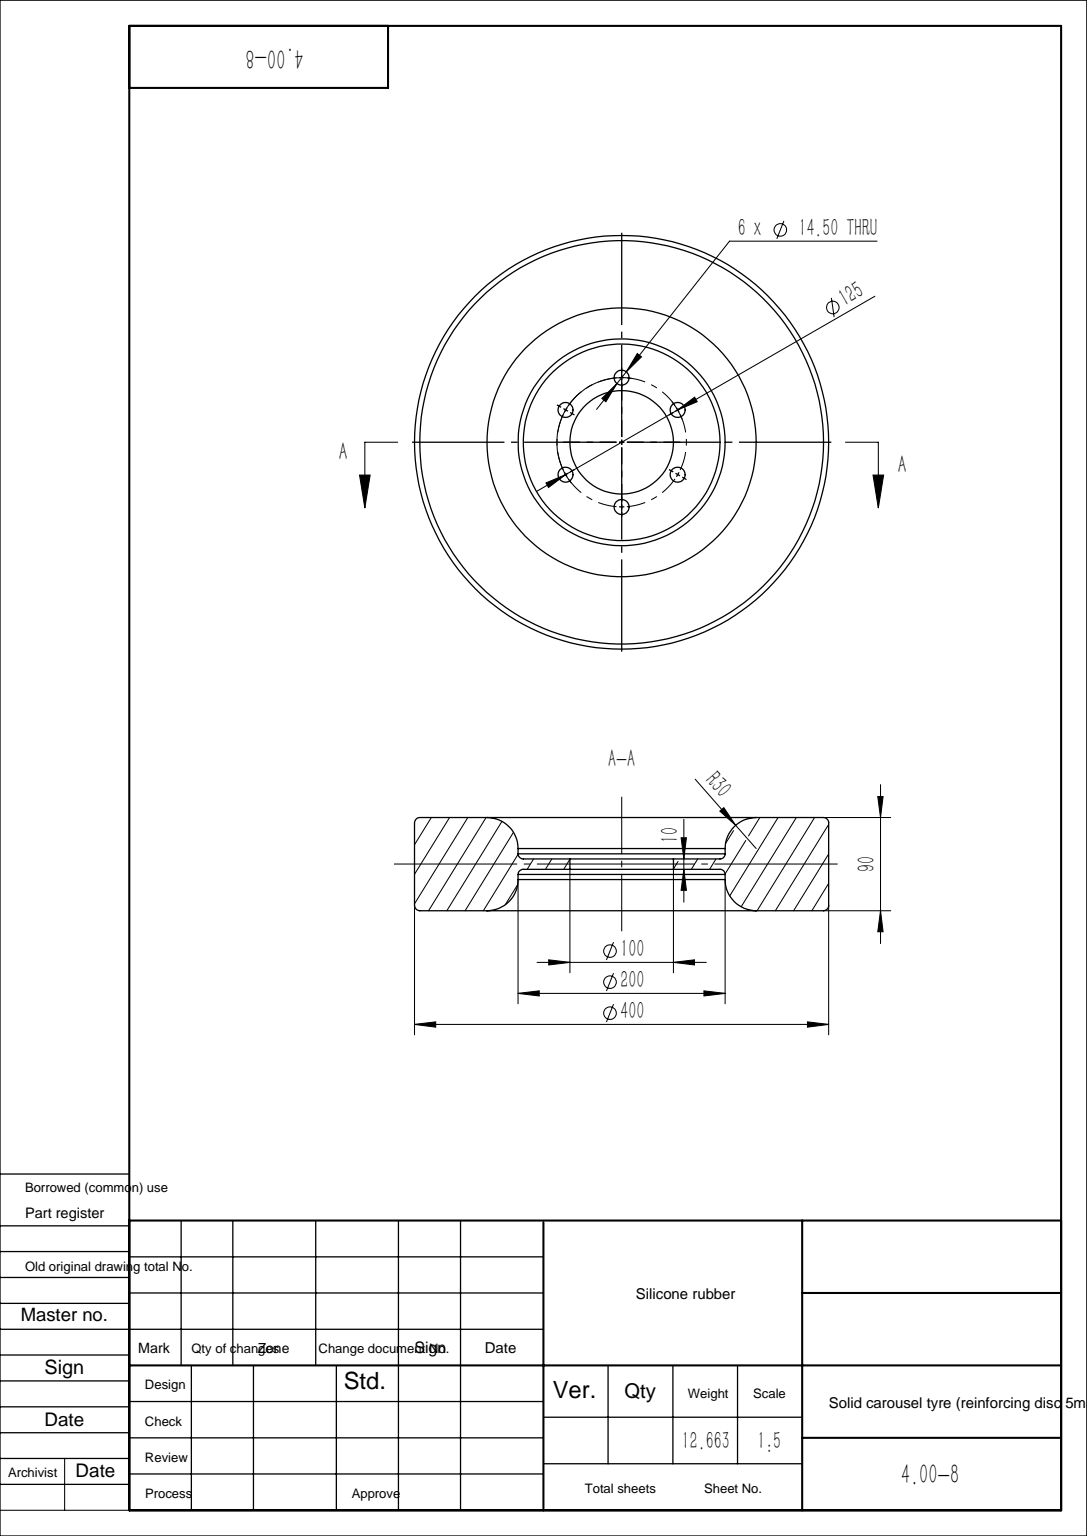
from build123d import *

# Parameters (mm, degrees)
FILLET1_R                    = 5
F_14_5_14_5_DIAMETER_HOLE1_D = 14.5


with BuildPart() as part:
    # Sketch2 → Revolve1 (revolve)
    with BuildSketch(Plane(origin=(0, 0, 0), x_dir=(1, 0, 0), z_dir=(0, 1, 0))):
        with BuildLine():
            Line((50, -5), (50, 5))
            Line((50, 5), (100, 5))
            Line((100, 5), (100, 15))
            ThreePointArc((100, 15), (108.786796564, 36.213203436), (130, 45))
            Line((130, 45), (200, 45))
            Line((200, 45), (200, -45))
            Line((200, -45), (130, -45))
            ThreePointArc((130, -45), (108.786796564, -36.213203436), (100, -15))
            Line((100, -15), (100, -5))
            Line((100, -5), (50, -5))
        make_face()
    revolve(axis=Axis((0, 0, 0), (0, 0, -1)))

    # Fillet1
    fillet1_edges = [part.edges().sort_by_distance(p)[0] for p in [
        (-100, 0, -5),
        (-100, 0, 5),
        (-200, 0, 45),
        (-200, 0, -45),
    ]]
    fillet(fillet1_edges, radius=FILLET1_R)

    # Ø14.5 (14.5) Diameter Hole1 (through all)
    with Locations(Plane.XY.offset(5)):
        with Locations((0, 62.5), (54.126587737, 31.25), (54.126587737, -31.25), (0, -62.5), (-54.126587737, -31.25), (-54.126587737, 31.25)):
            Hole(F_14_5_14_5_DIAMETER_HOLE1_D / 2)


solid = part.part
